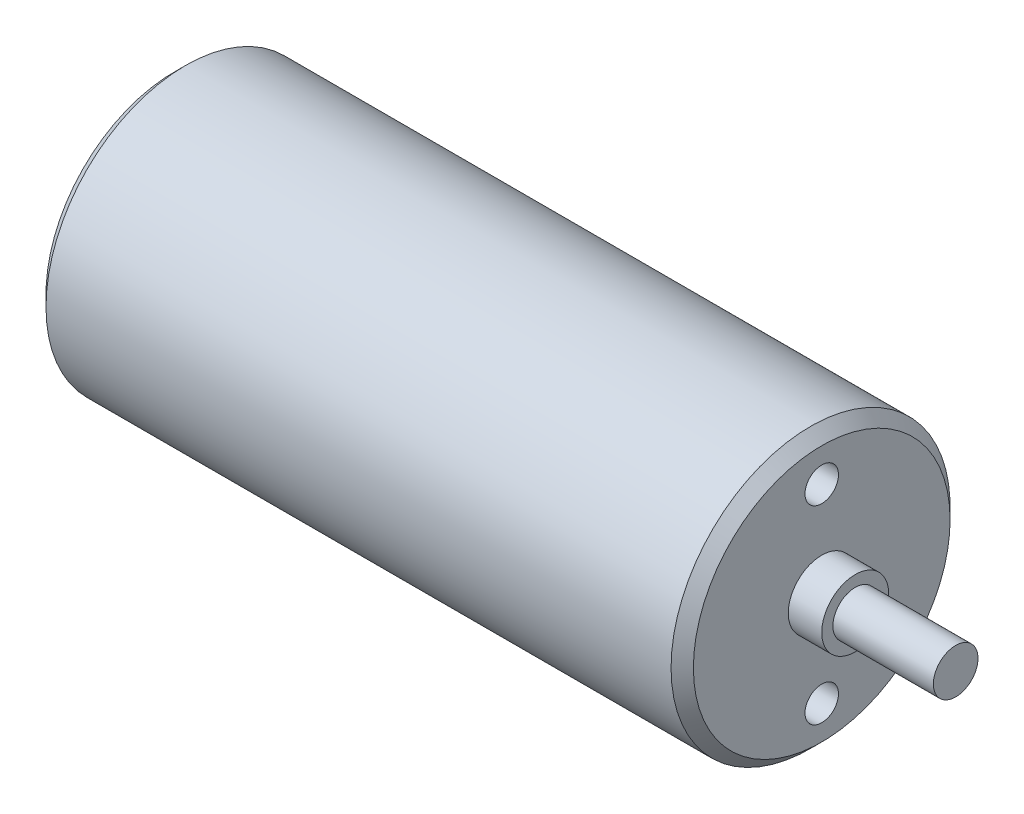
SolidWorks part; units mm, degrees
ref_plane "Front Plane" through (0, 0, 0) normal (0, 0, 1) x (1, 0, 0)
ref_plane "Top Plane" through (0, 0, 0) normal (0, 1, 0) x (1, 0, 0)
ref_plane "Right Plane" through (0, 0, 0) normal (1, 0, 0) x (0, 0, -1)
other "Configuration Table"
sketch "Sketch1" plane through (0, 0, 0) normal (1, 0, 0) x (0, 0, -1)
  circle A0 centre (0, 0) radius 12.5
  dimension "D1" = 25
extrude "Boss-Extrude1" add sketch "Sketch1" along normal blind 58
sketch "Sketch2" plane through (58, 0, 0) normal (1, 0, 0) x (0, 0, -1)
  circle A0 centre (0, 0) radius 3
  dimension "D1" = 6
extrude "Boss-Extrude2" add sketch "Sketch2" along normal blind 3
sketch "Sketch3" plane through (61, 0, 0) normal (1, 0, 0) x (0, 0, -1)
  circle A0 centre (0, 0) radius 2
  dimension "D1" = 4
extrude "Boss-Extrude3" add sketch "Sketch3" along normal blind 9
sketch "Sketch4" plane through (58, 0, 0) normal (1, 0, 0) x (0, 0, -1)
  line L0 (0, 0) -> (-6.3468, 0) construction
  circle A0 centre (0, 0) radius 8.5 construction
  circle A1 centre (0, 8.5) radius 1.5
  circle A2 centre (0, -8.5) radius 1.5
  dimension "D1" = 17
  dimension "D2" = 3
extrude "Cut-Extrude1" cut sketch "Sketch4" against normal blind 6
chamfer "Chamfer1" distance 1 angle 45 1 edges at (58, 0, -12.5)
chamfer "Chamfer2" distance 1 angle 45 1 edges at (0, 0, -12.5)
